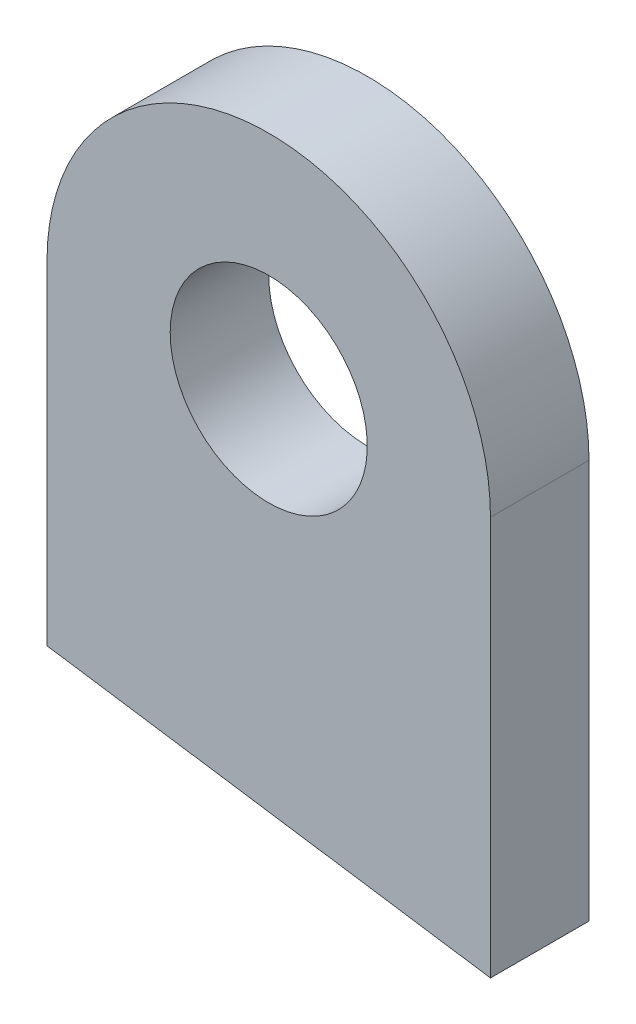
SolidWorks part; units mm, degrees
material "普通碳钢"
ref_plane "前视" through (0, 0, 0) normal (0, 0, 1) x (1, 0, 0)
ref_plane "上视" through (0, 0, 0) normal (0, 1, 0) x (1, 0, 0)
ref_plane "右视" through (0, 0, 0) normal (1, 0, 0) x (0, 0, -1)
sketch "草图1" plane through (0, 0, 0) normal (0, 0, 1) x (1, 0, 0)
  line L0 (-392.6885, 0) -> (384.1311, 0) construction
  line L1 (0, 300.9344) -> (0, -312.3443) construction
  line L2 (0, 0) -> (0, 81)
  line L6 (-90, 81) -> (-90, 13.3835)
  line L7 (-90, 13.3835) -> (0, 0)
  arc A0 (0, 81) -> (-90, 81) centre (-45, 81) ccw
  dimension "D6" = 81
  dimension "D2" = 90
  dimension "D1" = 73.5
  dimension "D4" = 90
extrude "凸台-拉伸1" add sketch "草图1" along normal blind 20
sketch "草图2" plane through (0, 0, 0) normal (0, 0, -1) x (-1, 0, 0)
  circle A0 centre (45, 81) radius 20
  dimension "D1" = 40
extrude "切除-拉伸1" cut sketch "草图2" against normal through all
